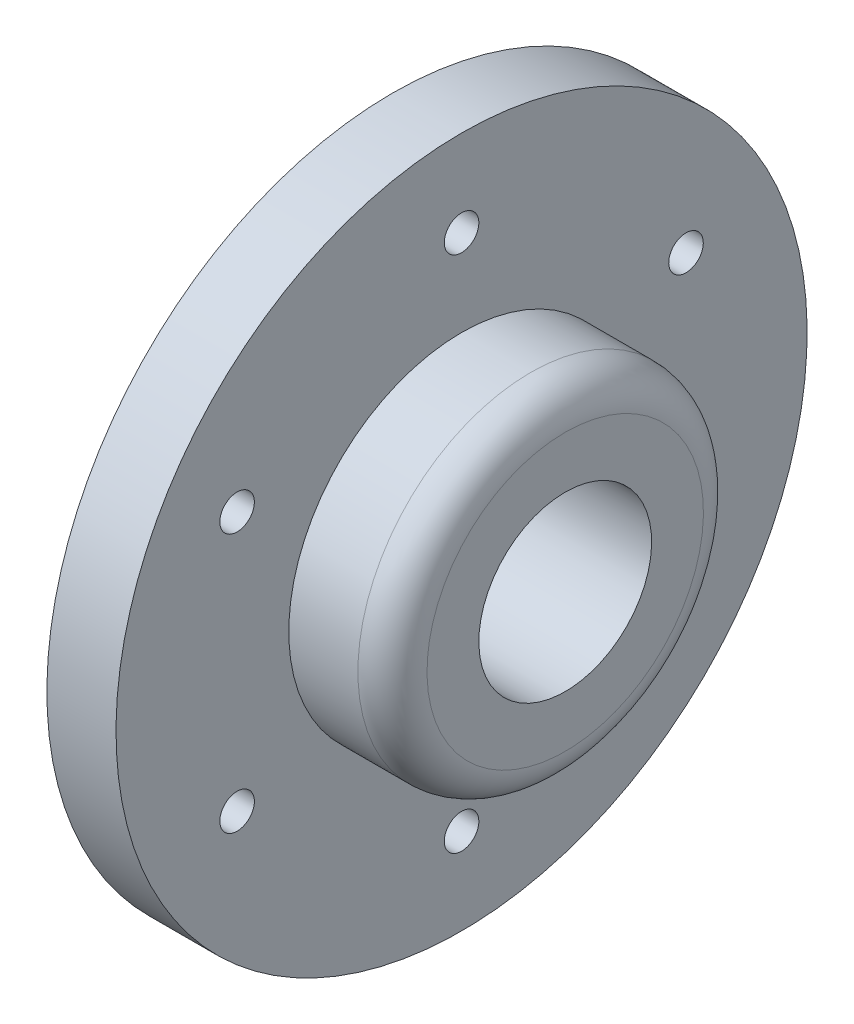
from build123d import *

# Parameters (mm, degrees)
CUT_EXTRUDE1_REACH = 146.568
SKETCH3_R          = 5
CIRPATTERN1_COUNT  = 6
FILLET1_R          = 10


with BuildPart() as part:
    # Sketch1 → Revolve1 (revolve)
    with BuildSketch(Plane.XY):
        Polygon((0, 25), (0, 100), (20, 100), (20, 50), (50, 50), (50, 25), align=None)
    revolve(axis=Axis((113.213850314, 0, 0), (-1, 0, 0)))

    # Sketch3 → Cut-Extrude1 (cut, up to next)
    with BuildSketch(Plane(origin=(20, 0, 0), x_dir=(0, 0, -1), z_dir=(1, 0, 0)), mode=Mode.PRIVATE) as cut_extrude1_sk1:
        with Locations(Location((0, 75, 0), (0, 0, 90))):
            Circle(SKETCH3_R)
    cut_extrude1_tool1 = extrude(cut_extrude1_sk1.sketch, amount=-CUT_EXTRUDE1_REACH, mode=Mode.PRIVATE) & part.part
    cut_extrude1 = cut_extrude1_tool1.solids().sort_by_distance((20, 75, 0))[0]
    add(cut_extrude1, mode=Mode.SUBTRACT)

    # CirPattern1: Cut-Extrude1 ×6 about axis
    cirpattern1_axis = Axis((0, 0, 0), (1, 0, 0))
    for i in range(1, CIRPATTERN1_COUNT):
        add(cut_extrude1.rotate(cirpattern1_axis, i * 360 / CIRPATTERN1_COUNT), mode=Mode.SUBTRACT)

    # Fillet1
    fillet1_edges = [part.edges().sort_by_distance(p)[0] for p in [
        (50, -50, 0),
    ]]
    fillet(fillet1_edges, radius=FILLET1_R)


solid = part.part
